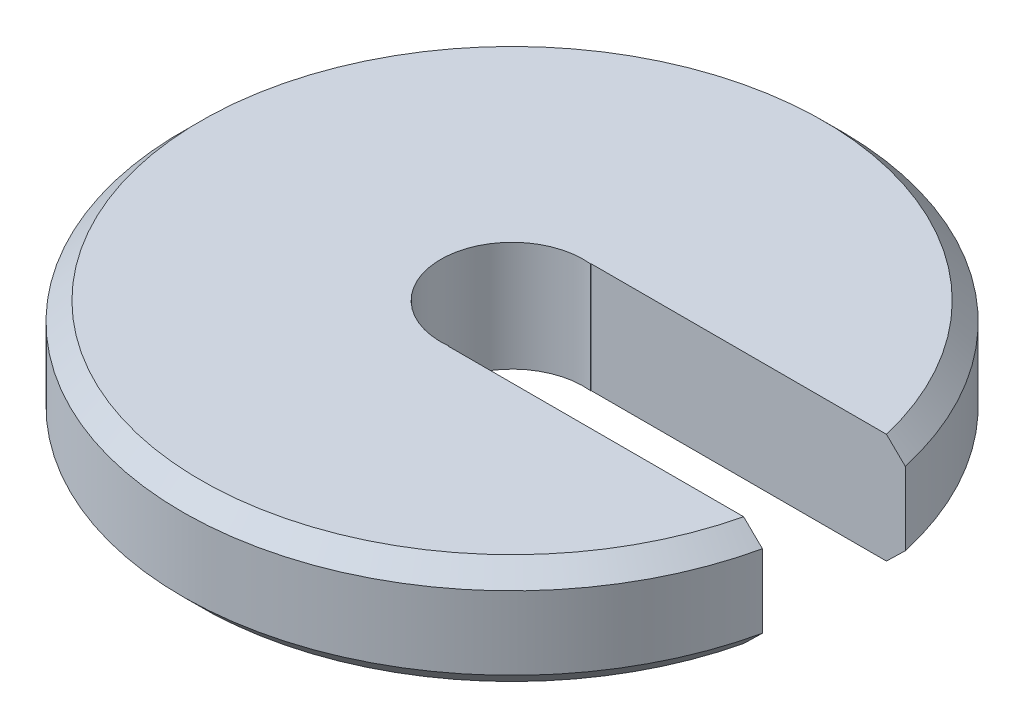
from build123d import *

# Parameters (mm, degrees)
SKETCH1_R           = 30
BOSS_EXTRUDE1_DEPTH = 10
SKETCH2_W           = 58.621984262
SKETCH2_H           = 13
CUT_EXTRUDE1_DEPTH  = 33
SKETCH3_R           = 6.5
CUT_EXTRUDE2_DEPTH  = 33
CHAMFER1_SIZE       = 1.67


with BuildPart() as part:
    # Sketch1 → Boss-Extrude1 (new body)
    with BuildSketch(Plane(origin=(0, 0, 0), x_dir=(1, 0, 0), z_dir=(0, 1, 0))):
        with Locations(Location((0, 0, 0), (0, 0, 270))):
            Circle(SKETCH1_R)
    extrude(amount=BOSS_EXTRUDE1_DEPTH)

    # Sketch2 → Cut-Extrude1 (cut)
    with BuildSketch(Plane(origin=(0, 10, 0), x_dir=(1, 0, 0), z_dir=(0, 1, 0))):
        with Locations((30, 0)):
            Rectangle(SKETCH2_W, SKETCH2_H)
    extrude(amount=-CUT_EXTRUDE1_DEPTH, mode=Mode.SUBTRACT)

    # Sketch3 → Cut-Extrude2 (cut)
    with BuildSketch(Plane(origin=(0, 10, 0), x_dir=(1, 0, 0), z_dir=(0, 1, 0))):
        Circle(SKETCH3_R)
    extrude(amount=-CUT_EXTRUDE2_DEPTH, mode=Mode.SUBTRACT)

    # Chamfer1
    chamfer1_edges = [part.edges().sort_by_distance(p)[0] for p in [
        (-30, 0, 0),
        (-30, 10, 0),
    ]]
    chamfer(chamfer1_edges, length=CHAMFER1_SIZE)


solid = part.part
